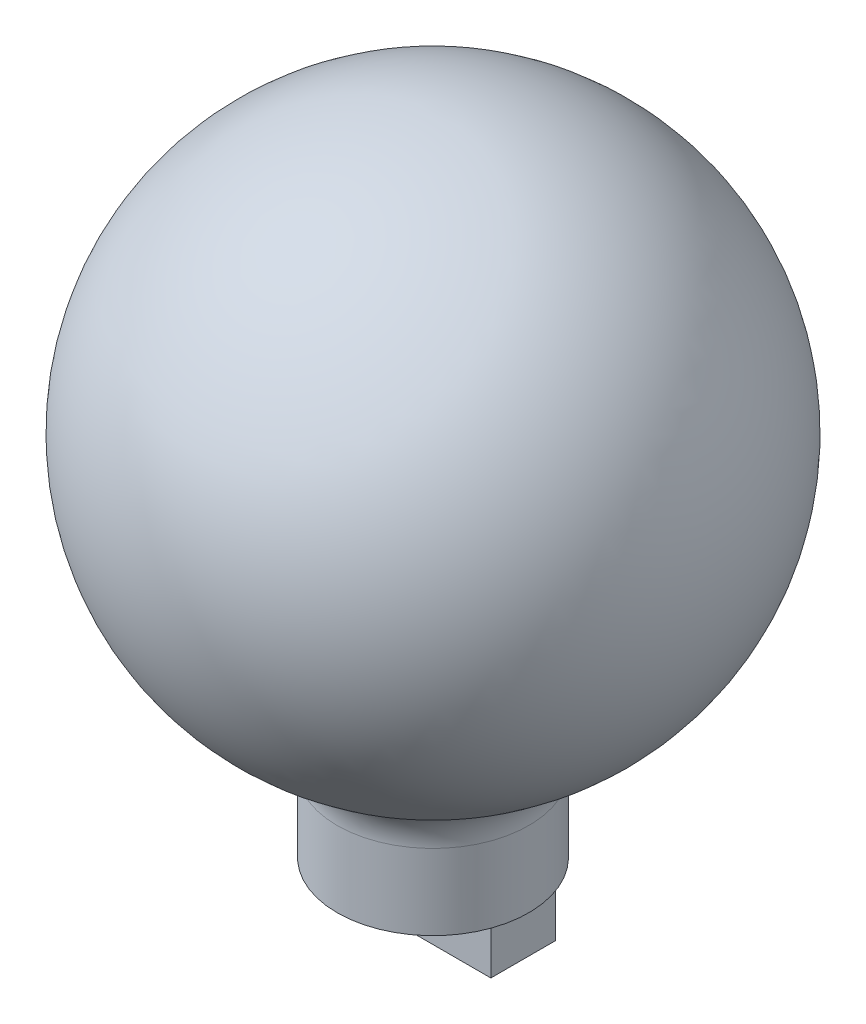
from build123d import *

# Parameters (mm, degrees)
SKETCH2_W               = 4.445
SKETCH2_H               = 19.05
FILETE2_R               = 2.54
SKETCH7_T_R             = 6.35
SKETCH7_T_R_2           = 2.5
CUT_EXTRUDE4_T_DEPTH    = 25.4
CUT_EXTRUDE1_DEPTH      = 27.181720795
CUT_EXTRUDE1_DEPTH_BACK = 27.181720795
SKETCH_1_W              = 15.700965646
SKETCH_1_H              = 4.620140609
SKETCH_2_W              = 8.368518388
SKETCH_2_H              = 3
BOSS_EXTRUDE1_DEPTH     = 2
SCALE1_SCALE            = 8.6


with BuildPart() as part:
    # Sketch1 → Revolve1 (revolve)
    with BuildSketch(Plane.XY):
        with BuildLine():
            Line((0, 12.7), (0, -12.7))
            ThreePointArc((0, -12.7), (-12.7, 0), (0, 12.7))
        make_face()
    revolve(axis=Axis((0, 12.7, 0), (0, -1, 0)))

    # Sketch2 → Revolve2 (revolve)
    with BuildSketch(Plane.XY, mode=Mode.PRIVATE) as revolve2_sk:
        with Locations((-2.2225, -9.525)):
            Rectangle(SKETCH2_W, SKETCH2_H)
    revolve(revolve2_sk.sketch.rotate(Axis((0, -19.05, 0), (0, 1, 0)), 180), axis=Axis((0, -19.05, 0), (0, 1, 0)))

    # Filete2
    filete2_edges = [part.edges().sort_by_distance(p)[0] for p in [
        (0, -11.896721187, 4.445),
    ]]
    fillet(filete2_edges, radius=FILETE2_R)

    # Sketch7-T → Cut-Extrude4-T (cut, symmetric)
    with BuildSketch(Plane(origin=(0, 0, 0), x_dir=(0, 0, -1), z_dir=(1, 0, 0))):
        with Locations((0, -24.765)):
            Circle(SKETCH7_T_R)
        with Locations((0, -66.675)):
            Circle(SKETCH7_T_R_2)
    extrude(amount=CUT_EXTRUDE4_T_DEPTH, both=True, mode=Mode.SUBTRACT)

    # 草图1 → Cut-Extrude1 (cut, two sides: drawn at the far end of the back side and taken through both)
    with BuildSketch(Plane(origin=(0, 0, 0), x_dir=(0, 0, -1), z_dir=(1, 0, 0)).offset(-CUT_EXTRUDE1_DEPTH_BACK)):
        with Locations((-0.056566237, -19.360070304)):
            Rectangle(SKETCH_1_W, SKETCH_1_H)
    extrude(amount=CUT_EXTRUDE1_DEPTH + CUT_EXTRUDE1_DEPTH_BACK, mode=Mode.SUBTRACT)


with BuildPart() as body_2:
    # 草图2 → Boss-Extrude1 (new body)
    with BuildSketch(Plane.XZ.offset(17.05)):
        Rectangle(SKETCH_2_W, SKETCH_2_H)
    extrude(amount=BOSS_EXTRUDE1_DEPTH)


with BuildPart() as part_1:
    # Scale1: scaled about (0, 0, 0)
    add(part.part.scale(SCALE1_SCALE))


with BuildPart() as body_2_1:
    # Scale1: scaled about (0, 0, 0)
    add(body_2.part.scale(SCALE1_SCALE))


solid = Compound([part_1.part, body_2_1.part])
